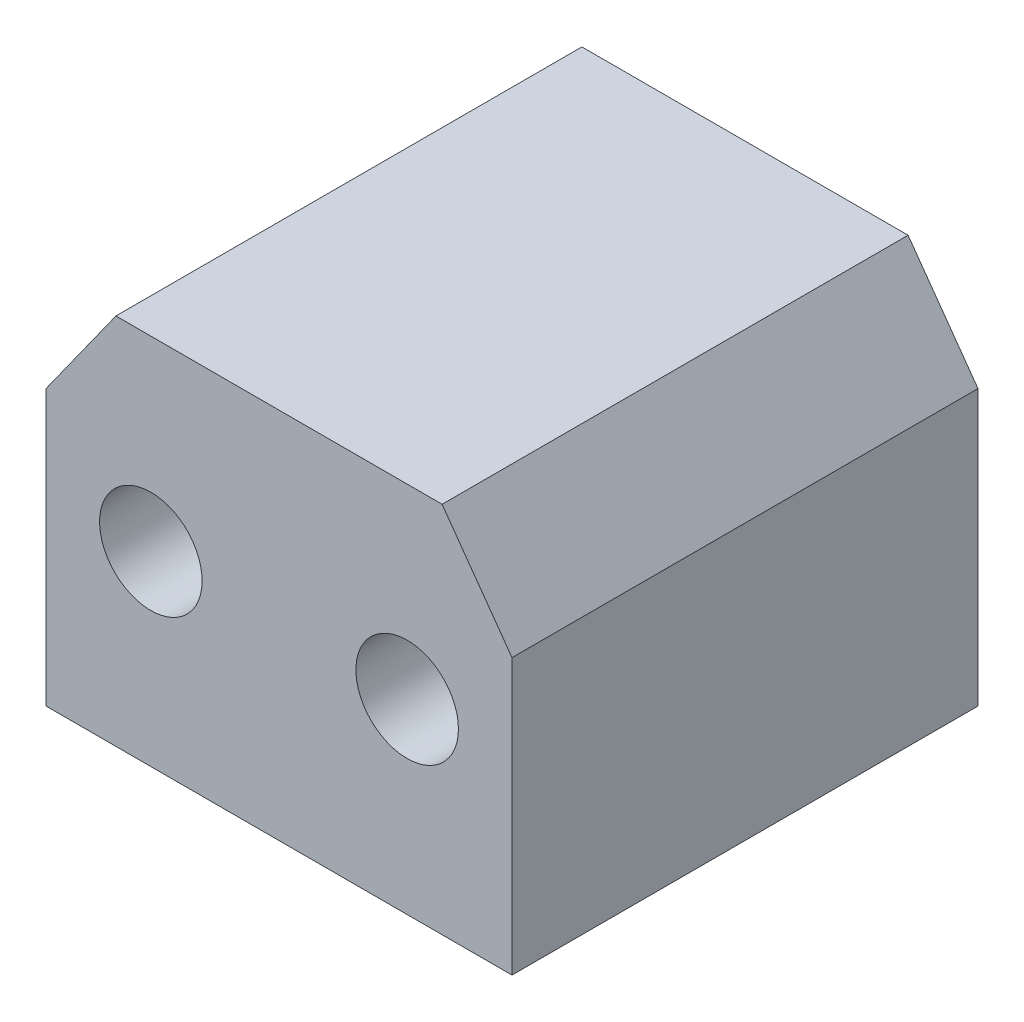
from build123d import *

# Parameters (mm, degrees)
SKETCH1_W               = 100
SKETCH1_H               = 80
BOSS_EXTRUDE1_DEPTH     = 100
CHAMFER1_SIZE           = 10
F_22_DIAMETER_HOLE1_D   = 22
CUT_EXTRUDE1_DEPTH      = 119.74342087
CUT_EXTRUDE1_DEPTH_BACK = 119.74342087


with BuildPart() as part:
    # Sketch1 → Boss-Extrude1 (new body)
    with BuildSketch(Plane.XY):
        Rectangle(SKETCH1_W, SKETCH1_H)
    extrude(amount=BOSS_EXTRUDE1_DEPTH)

    # Chamfer1
    chamfer1_edges = [part.edges().sort_by_distance(p)[0] for p in [
        (-50, 40, 50),
        (50, 40, 50),
    ]]
    chamfer(chamfer1_edges, length=CHAMFER1_SIZE)

    # Ø22 diameter hole1 (through all)
    with Locations(Plane.XY.offset(100)):
        with Locations((-27.5, 0), (27.5, 0)):
            Hole(F_22_DIAMETER_HOLE1_D / 2)

    # Sketch4 → Cut-Extrude1 (cut, two sides: drawn at the far end of the back side and taken through both)
    with BuildSketch(Plane.XY.offset(100).offset(-CUT_EXTRUDE1_DEPTH_BACK)):
        Polygon((-35, 40), (-50, 19), (-50, 40), align=None)
        Polygon((50, 40), (35, 40), (50, 19), align=None)
    extrude(amount=CUT_EXTRUDE1_DEPTH + CUT_EXTRUDE1_DEPTH_BACK, mode=Mode.SUBTRACT)


solid = part.part
